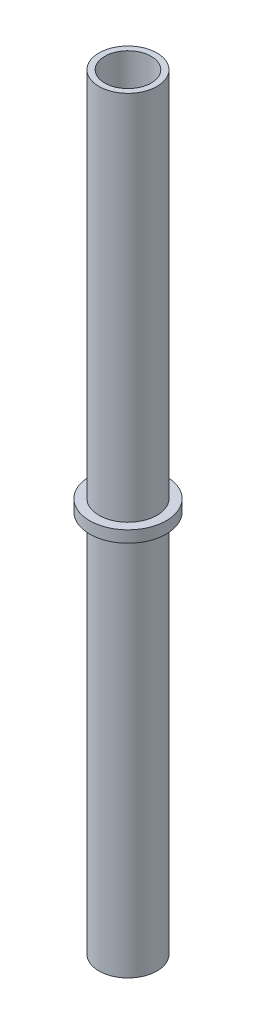
from build123d import *

# Parameters (mm, degrees)
SKETCH2_R          = 20
CUT_EXTRUDE1_DEPTH = 662.64794264


with BuildPart() as part:
    # Sketch1 → Revolve1 (revolve)
    with BuildSketch(Plane.XY, mode=Mode.PRIVATE) as revolve1_sk:
        Polygon((0, 0), (25, 0), (25, 330), (33, 330), (33, 340), (25, 340), (25, 585.119663834), (25, 619.032357738), (25, 660), (0, 660), align=None)
    revolve(revolve1_sk.sketch.rotate(Axis((0, 660, 0), (0, -1, 0)), 180), axis=Axis((0, 660, 0), (0, -1, 0)))

    # Sketch2 → Cut-Extrude1 (cut, through all)
    with BuildSketch(Plane(origin=(0, 660, 0), x_dir=(1, 0, 0), z_dir=(0, 1, 0))):
        with Locations(Location((0, 0, 0), (0, 0, 180))):
            Circle(SKETCH2_R)
    extrude(amount=-CUT_EXTRUDE1_DEPTH, mode=Mode.SUBTRACT)


solid = part.part
